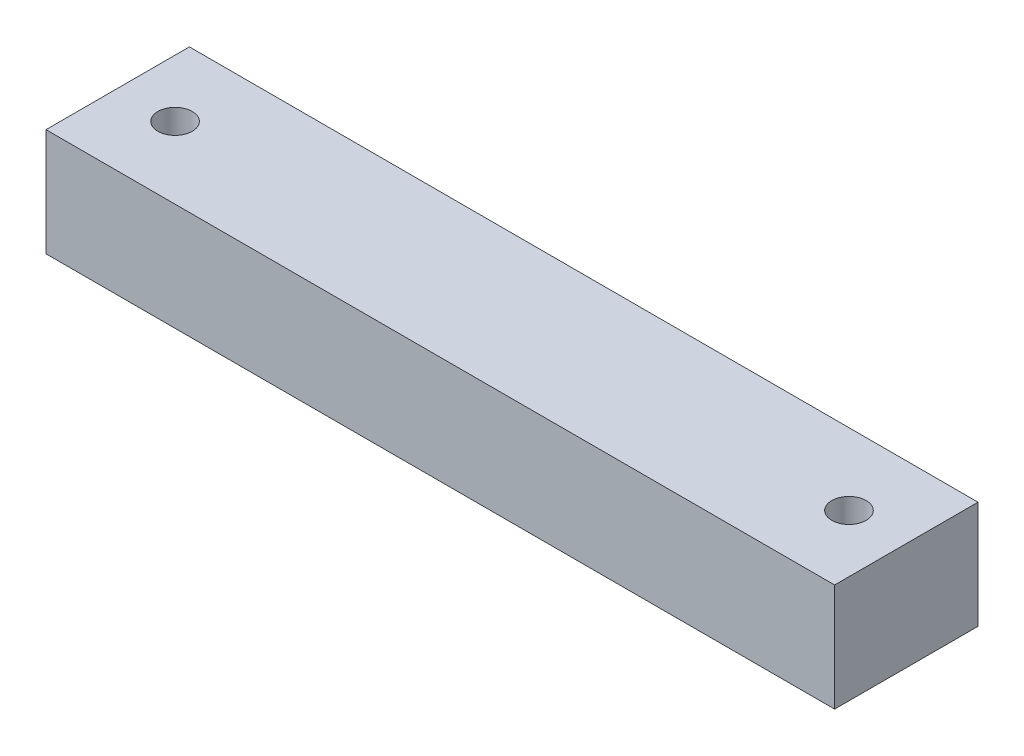
SolidWorks part; units mm, degrees
material "标准件"
ref_plane "前视基准面" through (0, 0, 0) normal (0, 0, 1) x (1, 0, 0)
ref_plane "上视基准面" through (0, 0, 0) normal (0, 1, 0) x (1, 0, 0)
ref_plane "右视基准面" through (0, 0, 0) normal (1, 0, 0) x (0, 0, -1)
sketch "草图1" plane through (0, 0, 0) normal (0, 1, 0) x (1, 0, 0)
  line L1 (-55, -10) -> (55, -10)
  line L2 (-55, -10) -> (-55, 10)
  line L3 (-55, 10) -> (55, 10)
  line L4 (55, -10) -> (55, 10)
  line L5 (-55, -10) -> (55, 10) construction
  line L6 (-55, 10) -> (55, -10) construction
  point P0 (0, 0)
  dimension "D1" = 110
  dimension "D2" = 20
extrude "凸台-拉伸1" add sketch "草图1" along normal blind 15
hole_wizard "M4 间隙孔1" positions "草图2" profile "草图3" hole size "M4" standard "ISO" end condition through all
sketch "草图2" plane through (0, 15, 0) normal (0, 1, 0) x (1, 0, 0)
  line L0 (0, 10) -> (0, -10) construction
  line L1 (55, 10) -> (-55, 10) construction
  line L2 (-55, -10) -> (55, -10) construction
  point P0 (-47, 0)
  point P2 (47, 0)
  dimension "D1" = 94
sketch "草图3" plane through (-47, 15, 0) normal (1, 0, 0) x (0, 0, 1)
  line L0 (0, 0) -> (0, 15)
  line L1 (0, 15) -> (2.4, 15)
  line L2 (2.4, 15) -> (2.4, 0)
  line L5 (2.4, 0) -> (0, 0)
  line L11 (0, -6.35) -> (0, 107.95) construction
  dimension "通孔孔直径" = 4.8
  dimension "通孔孔深度" = 15
